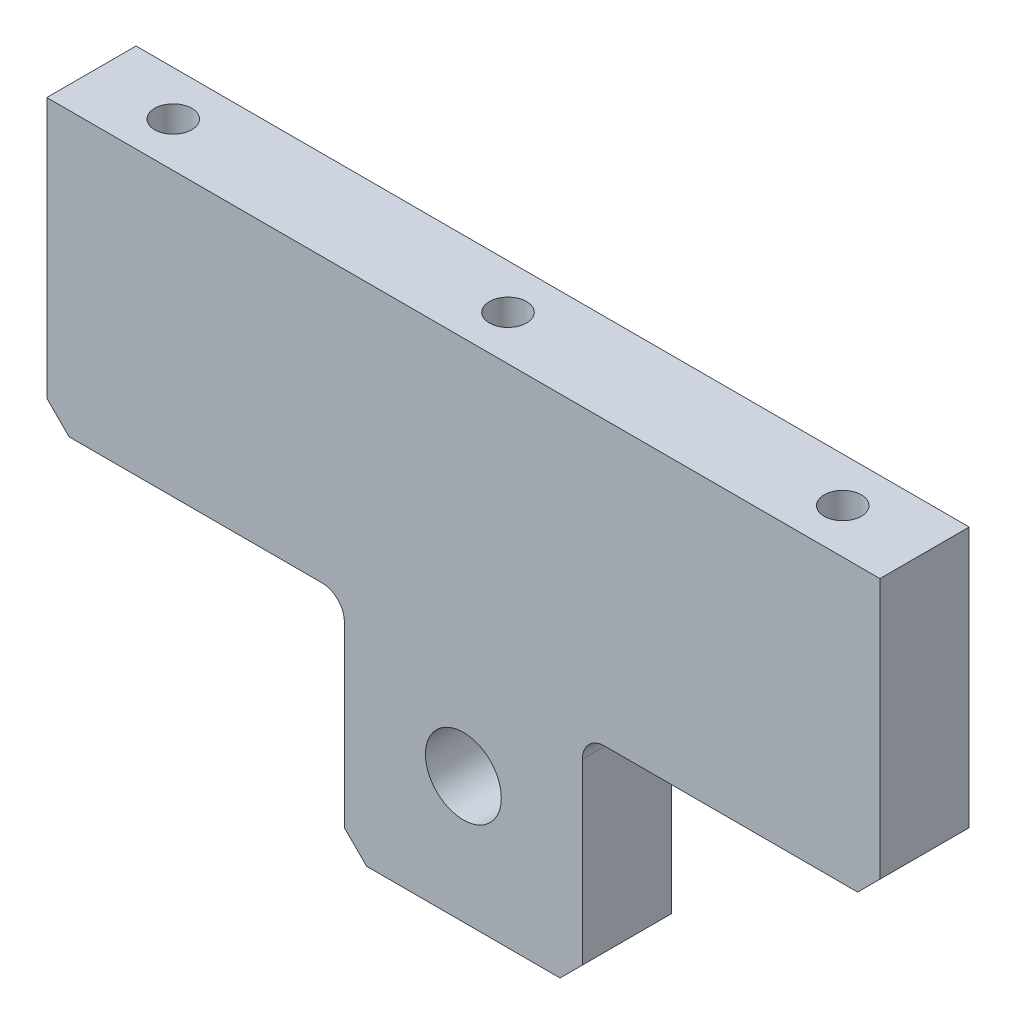
SolidWorks part; units mm, degrees
ref_plane "前视基准面" through (0, 0, 0) normal (0, 0, 1) x (1, 0, 0)
ref_plane "上视基准面" through (0, 0, 0) normal (0, 1, 0) x (1, 0, 0)
ref_plane "右视基准面" through (0, 0, 0) normal (1, 0, 0) x (0, 0, -1)
sketch "草图1" plane through (0, 0, 0) normal (0, 0, 1) x (1, 0, 0)
  line L1 (0, 0) -> (112, 0)
  line L2 (0, 0) -> (0, 68)
  line L3 (0, 68) -> (112, 68)
  line L4 (112, 0) -> (112, 68)
  dimension "D1" = 112
  dimension "D2" = 68
extrude "凸台-拉伸1" add sketch "草图1" along normal blind 12
sketch "草图2" plane through (0, 0, 12) normal (0, 0, 1) x (1, 0, 0)
  line L1 (0, 0) -> (40, 0)
  line L2 (0, 0) -> (0, 30)
  line L3 (0, 30) -> (40, 30)
  line L4 (40, 0) -> (40, 30)
  dimension "D1" = 40
  dimension "D2" = 30
extrude "切除-拉伸1" cut sketch "草图2" against normal blind 12
ref_plane "基准面1" through (56, 0, 0) normal (-1, 0, 0) x (0, 0, 1)
mirror "镜向1" about plane through (56, 0, 0) normal (-1, 0, 0) of "切除-拉伸1"
hole_wizard "M12 螺纹孔1" positions "草图4" profile "草图3" tap size "M12" standard "ISO" end condition through all
sketch "草图4" plane through (0, 0, 12) normal (0, 0, 1) x (1, 0, 0)
  line L0 (56, 0) -> (56, 44.1231) construction
  line L1 (40, 0) -> (72, 0) construction
  point P0 (56, 17)
  dimension "D1" = 17
sketch "草图3" plane through (56, 17, 12) normal (1, 0, 0) x (0, -1, 0)
  line L0 (0, 0) -> (0, 12)
  line L1 (0, 12) -> (5.1, 12)
  line L2 (5.1, 12) -> (5.1, 0)
  line L5 (5.1, 0) -> (0, 0)
  line L11 (0, -6.35) -> (0, 107.95) construction
  dimension "通孔螺纹孔钻头直径" = 10.2
  dimension "通孔螺纹孔钻头深度" = 12
cosmetic thread "孔螺蚊线1" parameters "D2"=12
chamfer "倒角1" distance 3 angle 45 4 edges at (112, 30, 6) (0, 30, 6) (72, 0, 6) (40, 0, 6)
fillet "圆角1" radius 3 2 edges at (72, 30, 6) (40, 30, 6)
hole_wizard "M6 螺纹孔1" positions "草图8" profile "草图7" tap size "M6" standard "ISO"
sketch "草图8" plane through (0, 68, 0) normal (0, 1, 0) x (1, 0, 0)
  line L0 (112, -6) -> (0, -6) construction
  line L1 (112, -12) -> (112, 0) construction
  line L2 (0, -12) -> (0, 0) construction
  line L4 (56, -12) -> (56, 0) construction
  line L5 (112, -12) -> (0, -12) construction
  line L6 (112, 0) -> (0, 0) construction
  point P0 (101, -6)
  point P2 (56, -6)
  point P4 (11, -6)
  dimension "D1" = 90
sketch "草图7" plane through (101, 68, 6) normal (1, 0, 0) x (0, 0, 1)
  line L0 (0, 0) -> (0, 16.5022)
  line L1 (0, 16.5022) -> (2.5, 15)
  line L2 (2.5, 15) -> (2.5, 0)
  line L5 (2.5, 0) -> (0, 0)
  line L10 (0, 16.5022) -> (-2.5, 15) construction
  line L11 (0, -6.35) -> (0, 107.95) construction
  dimension "螺纹孔钻头直径" = 5
  dimension "螺纹孔钻头深度" = 15
  dimension "导头角度" = 118
cosmetic thread "孔螺蚊线2" parameters "D1"=12, "D2"=6
cosmetic thread "孔螺蚊线3" parameters "D1"=12, "D2"=6
cosmetic thread "孔螺蚊线4" parameters "D1"=12, "D2"=6
hole_wizard "M5 螺纹孔1" positions "草图10" profile "草图9" tap size "M5" standard "ISO"
sketch "草图10" plane through (0, 0, 0) normal (0, -1, 0) x (-1, 0, 0)
  point P0 (-63.5, -6)
  point P3 (-48.5, -6)
sketch "草图9" plane through (63.5, 0, 6) normal (1, 0, 0) x (0, 0, -1)
  line L0 (0, 0) -> (0, 13.6618)
  line L1 (0, 13.6618) -> (2.1, 12.4)
  line L2 (2.1, 12.4) -> (2.1, 0)
  line L5 (2.1, 0) -> (0, 0)
  line L10 (0, 13.6618) -> (-2.1, 12.4) construction
  line L11 (0, -6.35) -> (0, 107.95) construction
  dimension "螺纹孔钻头直径" = 4.2
  dimension "螺纹孔钻头深度" = 12.4
  dimension "导头角度" = 118
cosmetic thread "孔螺蚊线5" parameters "D1"=10, "D2"=5
cosmetic thread "孔螺蚊线6" parameters "D1"=10, "D2"=5
